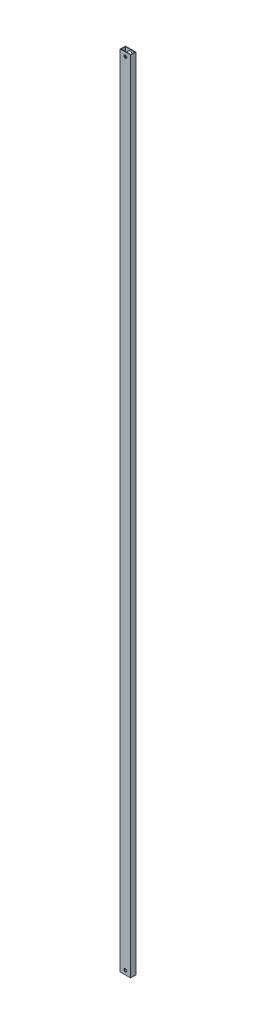
from build123d import *

# Parameters (mm, degrees)
SKETCH_2_W                = 20
SKETCH_2_H                = 10
SKETCH_2_W_2              = 18
SKETCH_2_H_2              = 8
EXTRUDE_1_DEPTH           = 1546.3
HOLE_WIZARD_1_D           = 5.5
HOLE_WIZARD_1_CBORE_D     = 10
HOLE_WIZARD_1_CBORE_DEPTH = 5.7


with BuildPart() as part:
    # 草图2 → 凸台-拉伸1 (new body)
    with BuildSketch(Plane(origin=(0, 0, 0), x_dir=(1, 0, 0), z_dir=(0, 1, 0))):
        Rectangle(SKETCH_2_W, SKETCH_2_H)
        Rectangle(SKETCH_2_W_2, SKETCH_2_H_2, mode=Mode.SUBTRACT)
    extrude(amount=EXTRUDE_1_DEPTH)

    # 打孔尺寸(%根据)内六角圆柱头螺钉的类型1 (through all)
    with Locations(Plane(origin=(0, 0, -5), x_dir=(-1, 0, 0), z_dir=(0, 0, -1))):
        with Locations((0, 1538.3), (0, 8)):
            CounterBoreHole(HOLE_WIZARD_1_D / 2, HOLE_WIZARD_1_CBORE_D / 2, HOLE_WIZARD_1_CBORE_DEPTH)


solid = part.part
